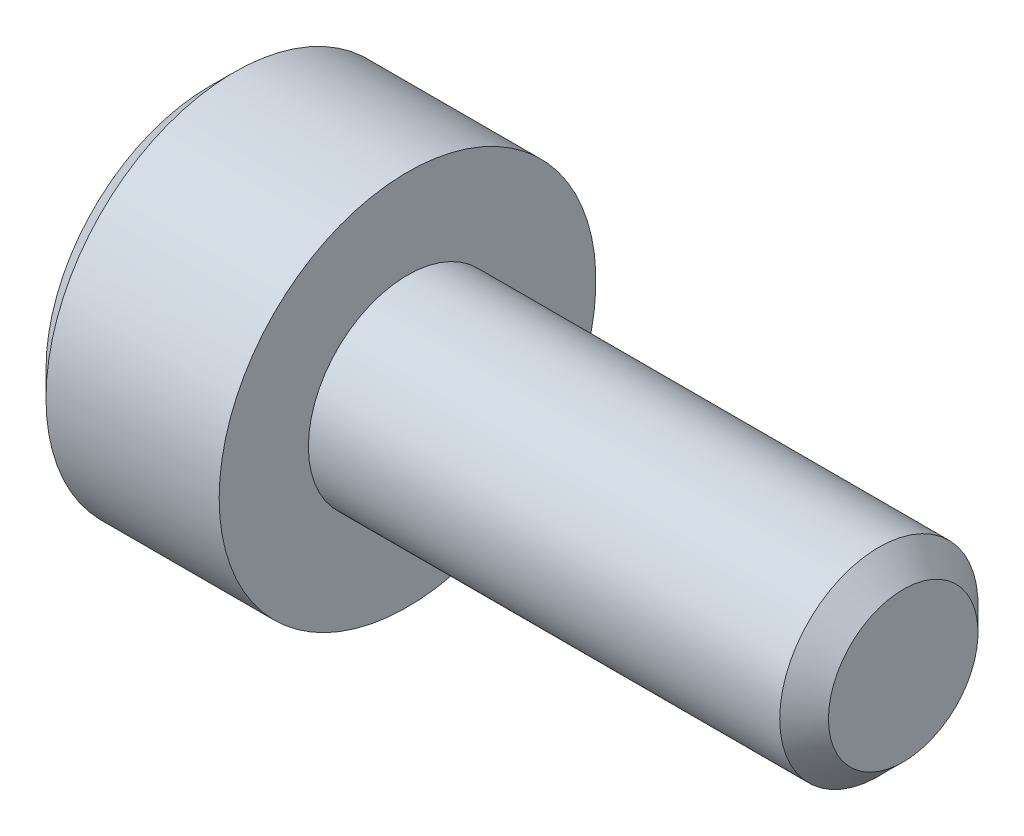
from build123d import *

# Parameters (mm, degrees)
CUT_EXTRUDE1_DEPTH = 1


with BuildPart() as part:
    # Sketch1 → Revolve1 (revolve)
    with BuildSketch(Plane.XY, mode=Mode.PRIVATE) as revolve1_sk:
        Polygon((-2, 0), (-2, 1.646666667), (-1.746666667, 1.9), (0, 1.9), (0, 1), (4.754266, 1), (5, 0.754266), (5, 0), align=None)
    revolve(revolve1_sk.sketch.rotate(Axis((5, 0, 0), (-1, 0, 0)), 270), axis=Axis((5, 0, 0), (-1, 0, 0)))

    # Sketch2 → Cut-Revolve1 (revolve, cut)
    with BuildSketch(Plane.XY, mode=Mode.PRIVATE) as cut_revolve1_sk:
        Polygon((-2, 0), (-2, 0.75), (-1, 0.75), (-0.799038106, 0), align=None)
    revolve(cut_revolve1_sk.sketch.rotate(Axis((-0.799038106, 0, 0), (-1, 0, 0)), 270), axis=Axis((-0.799038106, 0, 0), (-1, 0, 0)), mode=Mode.SUBTRACT)

    # Sketch3 → Cut-Extrude1 (cut)
    with BuildSketch(Plane(origin=(-2, 0, 0), x_dir=(0, 0, -1), z_dir=(1, 0, 0))):
        Polygon((-0.75, 0.433012702), (-0.75, -0.433012702), (0, -0.866025404), (0.75, -0.433012702), (0.75, 0.433012702), (0, 0.866025404), align=None)
    extrude(amount=CUT_EXTRUDE1_DEPTH, mode=Mode.SUBTRACT)


solid = part.part
